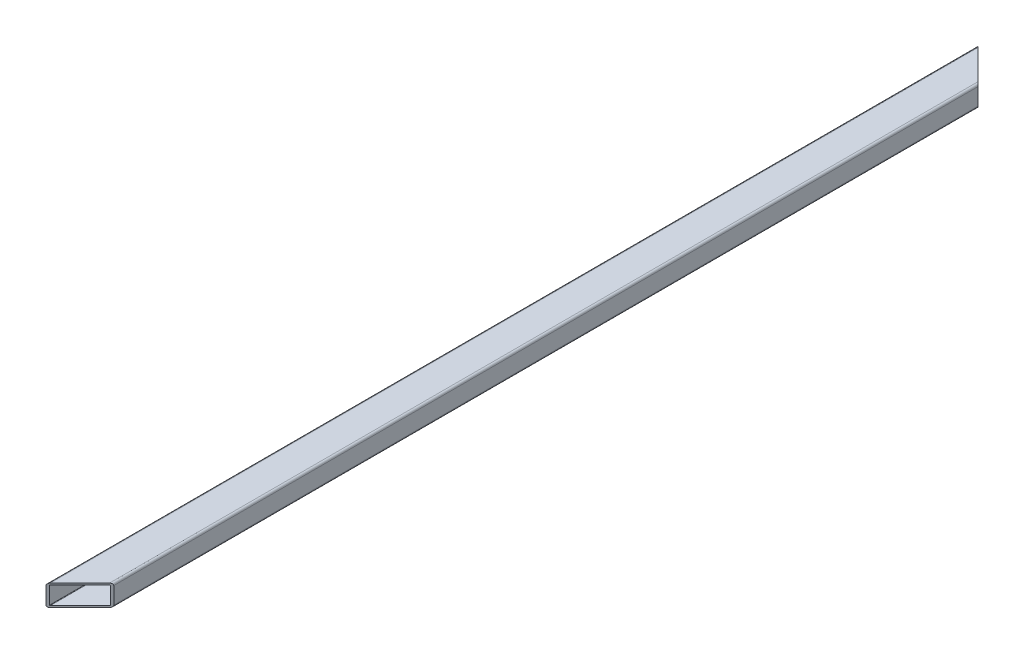
from build123d import *

# Parameters (mm, degrees)
BOSS_EXTRUDE1_DEPTH = 2200
SHELL1_T            = -4
CUT_EXTRUDE2_DEPTH  = 2000


with BuildPart() as part:
    # Sketch1 → Boss-Extrude1 (new body)
    with BuildSketch(Plane.XY):
        with BuildLine():
            Line((35, 25), (-35, 25))
            ThreePointArc((-35, 25), (-38.535533906, 23.535533906), (-40, 20))
            Line((-40, 20), (-40, -20))
            ThreePointArc((-40, -20), (-38.535533906, -23.535533906), (-35, -25))
            Line((-35, -25), (35, -25))
            ThreePointArc((35, -25), (38.535533906, -23.535533906), (40, -20))
            Line((40, -20), (40, 20))
            ThreePointArc((40, 20), (38.535533906, 23.535533906), (35, 25))
        make_face()
    extrude(amount=BOSS_EXTRUDE1_DEPTH)

    # Shell1
    shell1_openings = [part.faces().sort_by_distance(p)[0] for p in [
        (0, 0, 2200),
        (0, 0, 0),
    ]]
    offset(amount=SHELL1_T, openings=shell1_openings, kind=Kind.INTERSECTION)

    # Sketch3 → Cut-Extrude2 (cut)
    with BuildSketch(Plane.XZ.offset(25)):
        Polygon((-40, 2200), (40, 2120), (40, 2200), align=None)
        Polygon((40, 80), (40, 0), (-40, 0), align=None)
    extrude(amount=-CUT_EXTRUDE2_DEPTH, mode=Mode.SUBTRACT)


solid = part.part
